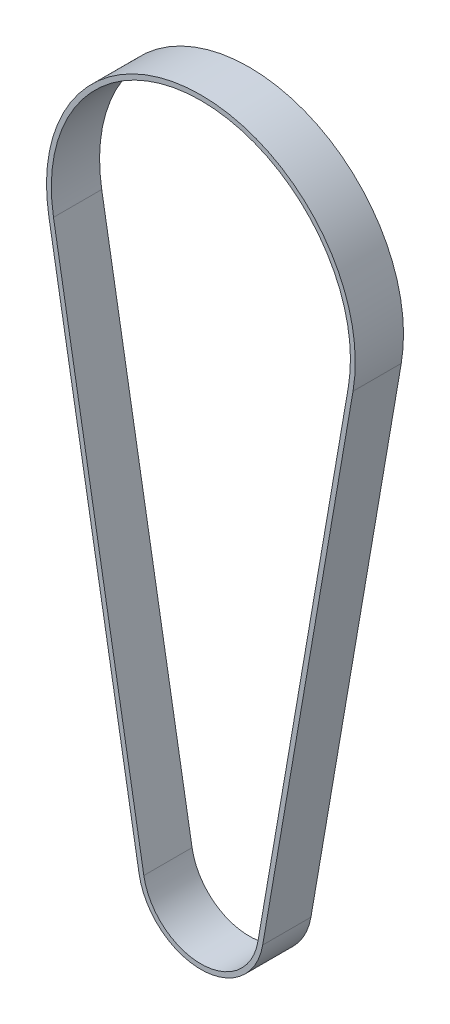
SolidWorks part; units mm, degrees
ref_plane "前视基准面" through (0, 0, 0) normal (0, 0, 1) x (1, 0, 0)
ref_plane "上视基准面" through (0, 0, 0) normal (0, 1, 0) x (1, 0, 0)
ref_plane "右视基准面" through (0, 0, 0) normal (1, 0, 0) x (0, 0, -1)
sketch "草图1" plane through (0, 0, 0) normal (0, 0, 1) x (1, 0, 0)
  line L0 (-62.0869, -10.6875) -> (-24.6376, -228.2411)
  line L1 (62.0869, -10.6875) -> (24.6376, -228.2411)
  arc A0 (62.0869, -10.6875) -> (-62.0869, -10.6875) centre (0, 0) ccw
  arc A1 (-24.6376, -228.2411) -> (24.6376, -228.2411) centre (0, -224) ccw
  dimension "D2" = 63
  dimension "D3" = 25
  dimension "D1" = 224
extrude "拉伸-薄壁1" add sketch "草图1" along normal blind 20 thin thin type two direction wall 1 second wall 1
